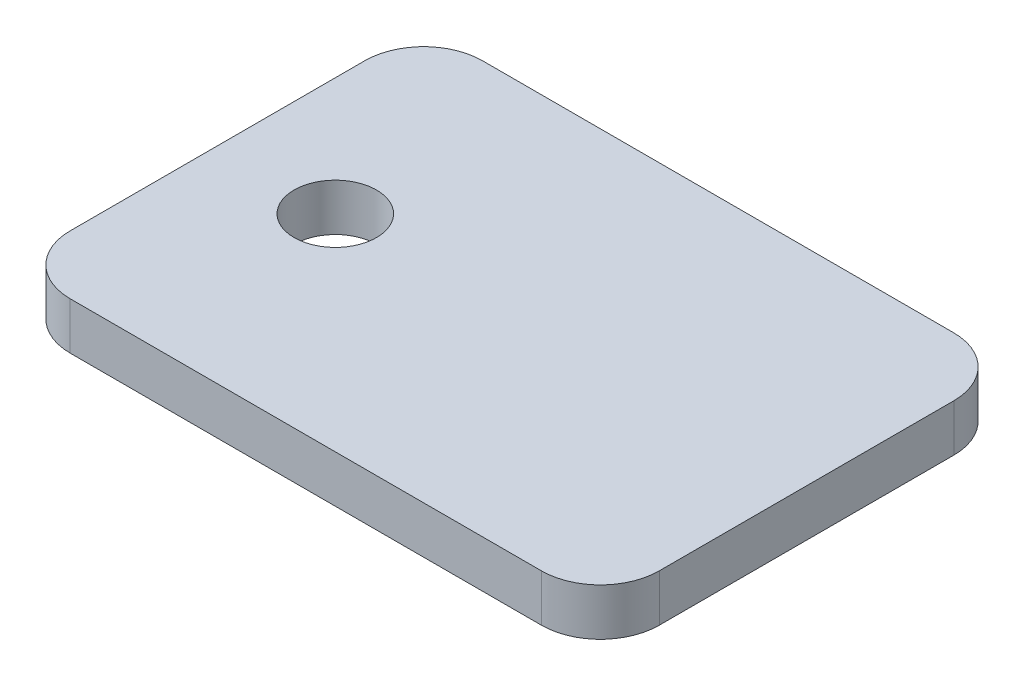
SolidWorks part; units mm, degrees
ref_plane "Front Plane" through (0, 0, 0) normal (0, 0, 1) x (1, 0, 0)
ref_plane "Top Plane" through (0, 0, 0) normal (0, 1, 0) x (1, 0, 0)
ref_plane "Right Plane" through (0, 0, 0) normal (1, 0, 0) x (0, 0, -1)
other "Configuration Table"
sketch "Sketch1" plane through (0, 0, 0) normal (0, 1, 0) x (1, 0, 0)
  line L1 (50, -35) -> (-50, -35)
  line L2 (50, -35) -> (50, 35)
  line L3 (50, 35) -> (-50, 35)
  line L4 (-50, -35) -> (-50, 35)
  line L5 (50, -35) -> (-50, 35) construction
  line L6 (50, 35) -> (-50, -35) construction
  point P0 (0, 0)
  dimension "D1" = 100
  dimension "D2" = 70
extrude "Boss-Extrude1" add sketch "Sketch1" along normal blind 8
fillet "Fillet1" radius 10 4 edges at (-50, 4, -35) (50, 4, -35) (50, 4, 35) (-50, 4, 35)
sketch "Sketch2" plane through (0, 8, 0) normal (0, 1, 0) x (1, 0, 0)
  line L0 (-50, 0) -> (50, 0) construction
  line L1 (-50, 25) -> (-50, -25) construction
  line L2 (50, -25) -> (50, 25) construction
  circle A0 centre (-30, 0) radius 7
  dimension "D1" = 14
  dimension "D2" = 20
extrude "Cut-Extrude1" cut sketch "Sketch2" against normal blind 8
